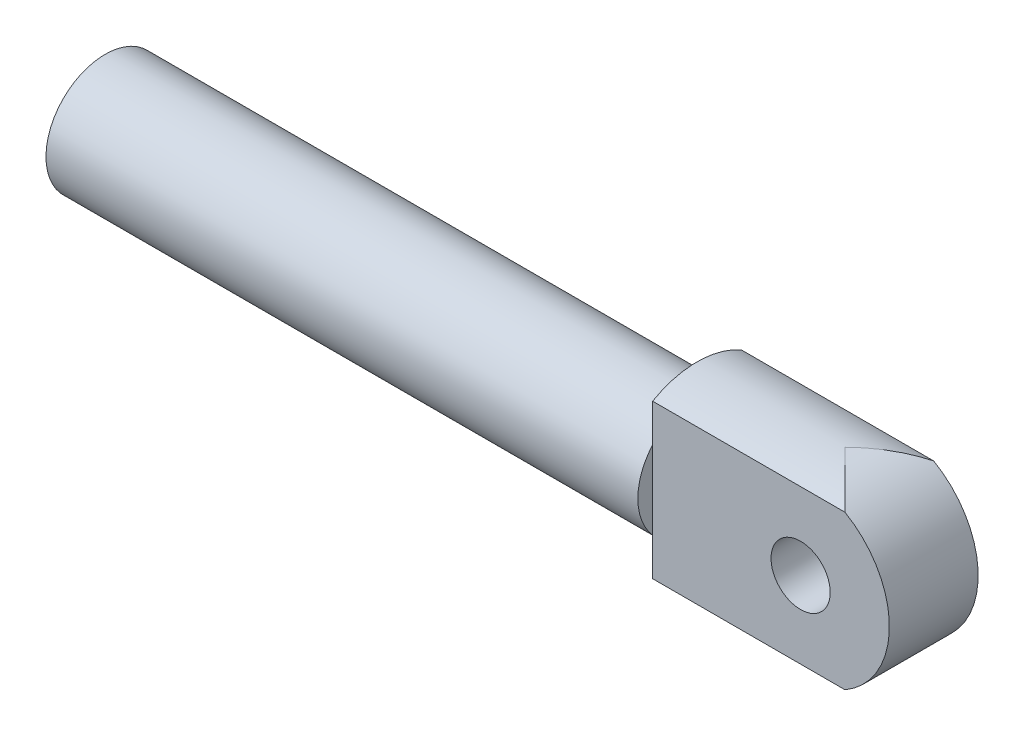
from build123d import *

# Parameters (mm, degrees)
SKETCH1_R               = 100
SKETCH1_R_2             = 50
BOSS_EXTRUDE1_DEPTH     = 1000
BOSS_EXTRUDE2_DEPTH     = 400
CUT_EXTRUDE2_DEPTH      = 1419.846362366
CUT_EXTRUDE2_DEPTH_BACK = 1419.846362366
CUT_EXTRUDE3_DEPTH      = 1419.846362366
CUT_EXTRUDE3_DEPTH_BACK = 1419.846362366
SKETCH_4_5_2_R          = 50


with BuildPart() as part:
    # Sketch1 → Boss-Extrude1 (new body)
    with BuildSketch(Plane(origin=(0, 0, 0), x_dir=(0, 0, -1), z_dir=(1, 0, 0))):
        Circle(SKETCH1_R)
        Circle(SKETCH1_R_2, mode=Mode.SUBTRACT)
    extrude(amount=BOSS_EXTRUDE1_DEPTH)

    # Sketch3 → Boss-Extrude2 (add)
    with BuildSketch(Plane(origin=(1000, 0, 0), x_dir=(0, 0, -1), z_dir=(1, 0, 0))):
        with BuildLine():
            Line((-75, 129.903810568), (-75, -129.903810568))
            ThreePointArc((-75, -129.903810568), (0, -150), (75, -129.903810568))
            Line((75, -129.903810568), (75, 129.903810568))
            ThreePointArc((75, 129.903810568), (0, 150), (-75, 129.903810568))
        make_face()
    extrude(amount=BOSS_EXTRUDE2_DEPTH)

    # Sketch 4_5 → Cut-Extrude2 (cut, two sides: drawn at the far end of the back side and taken through both)
    with BuildSketch(Plane.XY.offset(75).offset(-CUT_EXTRUDE2_DEPTH_BACK)):
        with BuildLine():
            Line((1250, 150), (1455.357524725, 150))
            Line((1455.357524725, 150), (1455.357524725, -150))
            Line((1455.357524725, -150), (1250, -150))
            ThreePointArc((1250, -150), (1400, 0), (1250, 150))
        make_face()
    extrude(amount=CUT_EXTRUDE2_DEPTH + CUT_EXTRUDE2_DEPTH_BACK, mode=Mode.SUBTRACT)

    # Sketch 4_5 2 → Cut-Extrude3 (cut, two sides: drawn at the far end of the back side and taken through both)
    with BuildSketch(Plane.XY.offset(75).offset(-CUT_EXTRUDE3_DEPTH_BACK)):
        with Locations((1250, 0)):
            Circle(SKETCH_4_5_2_R)
    extrude(amount=CUT_EXTRUDE3_DEPTH + CUT_EXTRUDE3_DEPTH_BACK, mode=Mode.SUBTRACT)


solid = part.part
